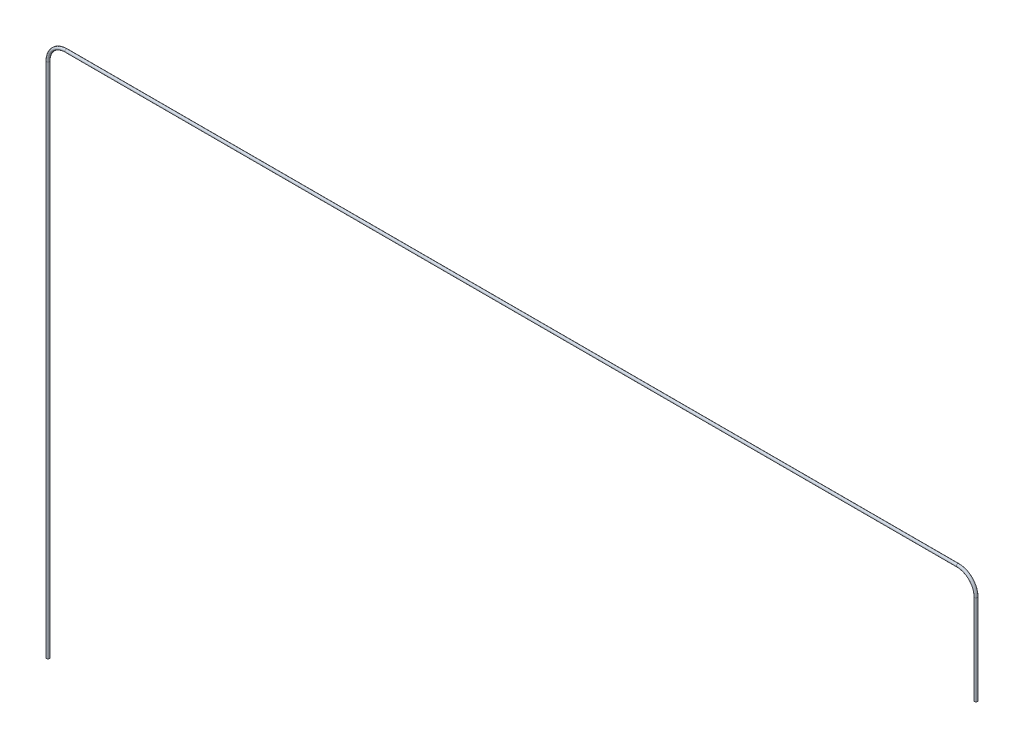
SolidWorks part; units mm, degrees
ref_plane "Front Plane" through (0, 0, 0) normal (0, 0, 1) x (1, 0, 0)
ref_plane "Top Plane" through (0, 0, 0) normal (0, 1, 0) x (1, 0, 0)
ref_plane "Right Plane" through (0, 0, 0) normal (1, 0, 0) x (0, 0, -1)
sketch "Sketch1" plane through (0, 0, 0) normal (0, 0, 1) x (1, 0, 0)
  line L0 (0, 0) -> (0, 1193)
  line L1 (42, 1235) -> (2100, 1235)
  line L2 (2142, 1193) -> (2142, 985)
  arc A0 (2100, 1235) -> (2142, 1193) centre (2100, 1193) cw
  arc A1 (0, 1193) -> (42, 1235) centre (42, 1193) cw
  point P7 (2142, 1235)
  point P10 (0, 1235)
  dimension "D3" = 42
  dimension "D1" = 2142
  dimension "D2" = 1235
  dimension "D4" = 250
sketch "Sketch2" plane through (0, 0, 0) normal (0, 1, 0) x (1, 0, 0)
  circle A0 centre (0, 0) radius 3.25
  dimension "D1" = 6.5
sweep "Sweep1" add profiles "Sketch2" path "Sketch1"
